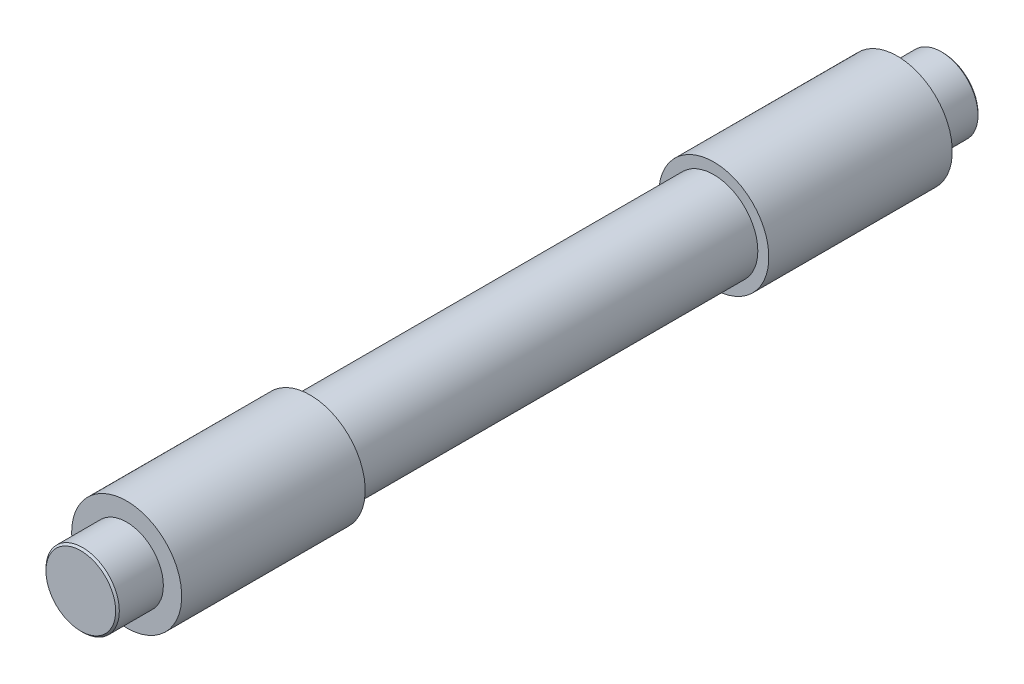
SolidWorks part; units mm, degrees
ref_plane "前视基准面" through (0, 0, 0) normal (0, 0, 1) x (1, 0, 0)
ref_plane "上视基准面" through (0, 0, 0) normal (0, 1, 0) x (1, 0, 0)
ref_plane "右视基准面" through (0, 0, 0) normal (1, 0, 0) x (0, 0, -1)
sketch "草图2" plane through (0, 0, 0) normal (0, 0, 1) x (1, 0, 0)
  circle A0 centre (0, 0) radius 30
extrude "凸台-拉伸1" add sketch "草图2" along normal blind 470
sketch "草图3" plane through (0, 0, 470) normal (0, 0, 1) x (1, 0, 0)
  circle A0 centre (0, 0) radius 20
  circle A3 centre (0, 0) radius 30
  circle A4 centre (0, 0) radius 30
  dimension "D1" = 0
extrude "切除-拉伸1" cut sketch "草图3" against normal blind 25
sketch "草图4" plane through (0, 0, 0) normal (0, 0, -1) x (-1, 0, 0)
  circle A0 centre (0, 0) radius 20
  circle A3 centre (0, 0) radius 30
  circle A4 centre (0, 0) radius 30
  dimension "D1" = 0
extrude "切除-拉伸2" cut sketch "草图4" against normal blind 25
sketch "草图5" plane through (0, 0, 0) normal (0, 1, 0) x (1, 0, 0)
  line L0 (-30, -25) -> (-30, -125)
  line L1 (-30, -25) -> (-30, -445) construction
  line L2 (-30, -445) -> (-30, -345)
  line L3 (-30, -345) -> (30, -345)
  line L4 (30, -445) -> (30, -25) construction
  line L5 (-30, -125) -> (-24, -125)
  line L6 (-24, -125) -> (-24, -345)
  line L7 (-30, -345) -> (-30, -125)
  line L8 (0, -345) -> (0, -325.8194)
revolve "切除-旋转1" cut sketch "草图5" angle 360 about L8
sketch "草图6" plane through (0, 0, 0) normal (0, 1, 0) x (1, 0, 0)
  line L0 (20, 0) -> (19, 0)
  line L1 (20, 0) -> (-20, 0) construction
  line L2 (20, 0) -> (20, -1)
  line L3 (20, -25) -> (20, 0) construction
  line L4 (20, -1) -> (19, 0)
  line L5 (24, -235) -> (43.7901, -235)
  line L6 (24, -345) -> (24, -125) construction
  line L8 (20, -469) -> (19, -470)
  line L9 (20, -470) -> (20, -469)
  line L10 (20, -470) -> (19, -470)
  line L11 (0, -470) -> (0, -466.0824)
  line L12 (-20, -470) -> (20, -470) construction
revolve "切除-旋转2" cut sketch "草图6" angle 360 about L11
